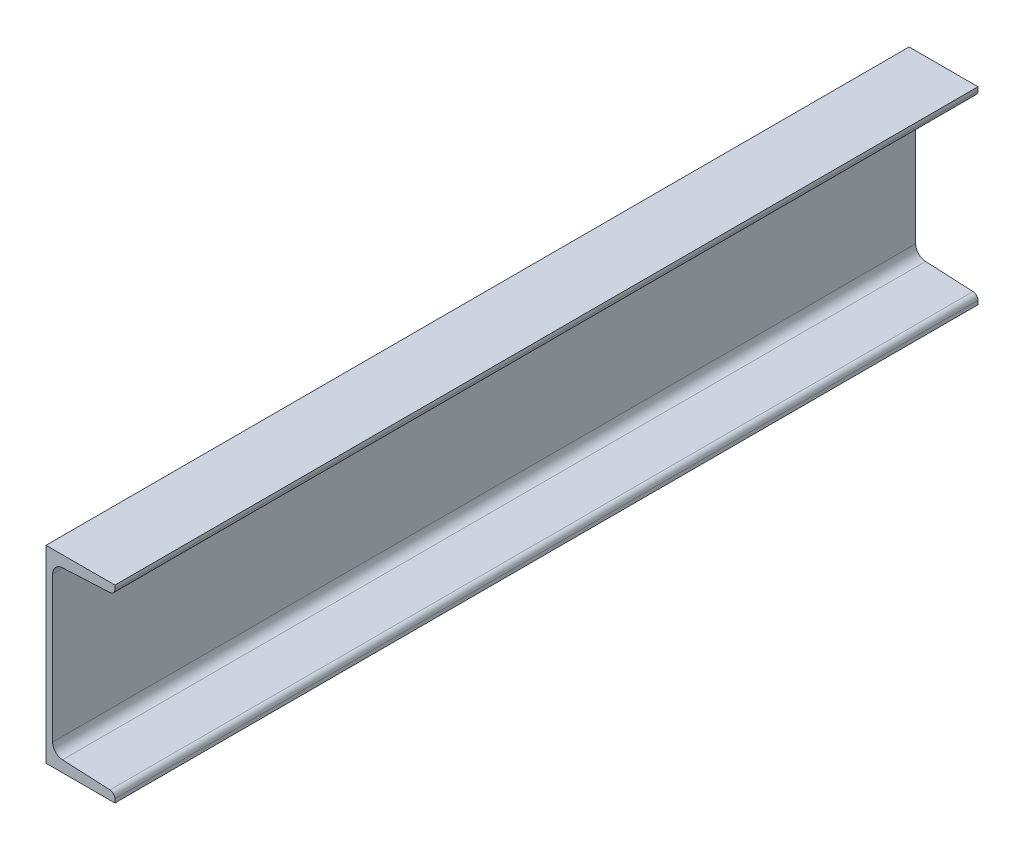
SolidWorks part; units mm, degrees
material "普通碳钢"
ref_plane "Front Plane" through (0, 0, 0) normal (0, 0, 1) x (1, 0, 0)
ref_plane "Top Plane" through (0, 0, 0) normal (0, 1, 0) x (1, 0, 0)
ref_plane "Right Plane" through (0, 0, 0) normal (1, 0, 0) x (0, 0, -1)
sketch "Sketch1" plane through (28.2113, 0, 0) normal (0, 0, 1) x (-1, 0, 0)
  line L0 (28.2113, 0) -> (28.2113, -200)
  line L1 (28.2113, -200) -> (-44.7887, -200)
  line L2 (28.2113, -100) -> (21.2113, -100) construction
  line L3 (21.2113, -177.0757) -> (21.2113, -22.9243)
  line L4 (10.7523, -188.0624) -> (-39.5592, -190.5398)
  line L5 (-44.7887, -196.0332) -> (-44.7887, -200)
  line L6 (21.2113, -187.5473) -> (21.2113, -190.7973) construction
  line L7 (21.2113, -190.7973) -> (-44.7887, -190.7973) construction
  line L8 (-8.2887, -200) -> (-8.2887, -189) construction
  line L9 (-44.7887, -3.9668) -> (-44.7887, 0)
  line L10 (28.2113, 0) -> (-44.7887, 0)
  line L11 (10.7523, -11.9376) -> (-39.5592, -9.4602)
  arc A0 (21.2113, -177.0757) -> (10.7523, -188.0624) centre (10.2113, -177.0757) cw
  arc A1 (10.7523, -11.9376) -> (21.2113, -22.9243) centre (10.2113, -22.9243) cw
  arc A2 (-39.5592, -190.5398) -> (-44.7887, -196.0332) centre (-39.2887, -196.0332) ccw
  arc A3 (-44.7887, -3.9668) -> (-39.5592, -9.4602) centre (-39.2887, -3.9668) ccw
  point P2 (-8.2887, 0)
  point P20 (21.2113, -12.4527)
  point P26 (-44.7887, -9.2027)
  dimension "r" = 11
  dimension "r1" = 5.5
  dimension "h" = 200
  dimension "b" = 73
  dimension "d" = 7
  dimension "t" = 11
  dimension "D5" = 66
  dimension "D6" = 3.25
extrude "Boss-Extrude1" add sketch "Sketch1" along normal mid plane 914.4
